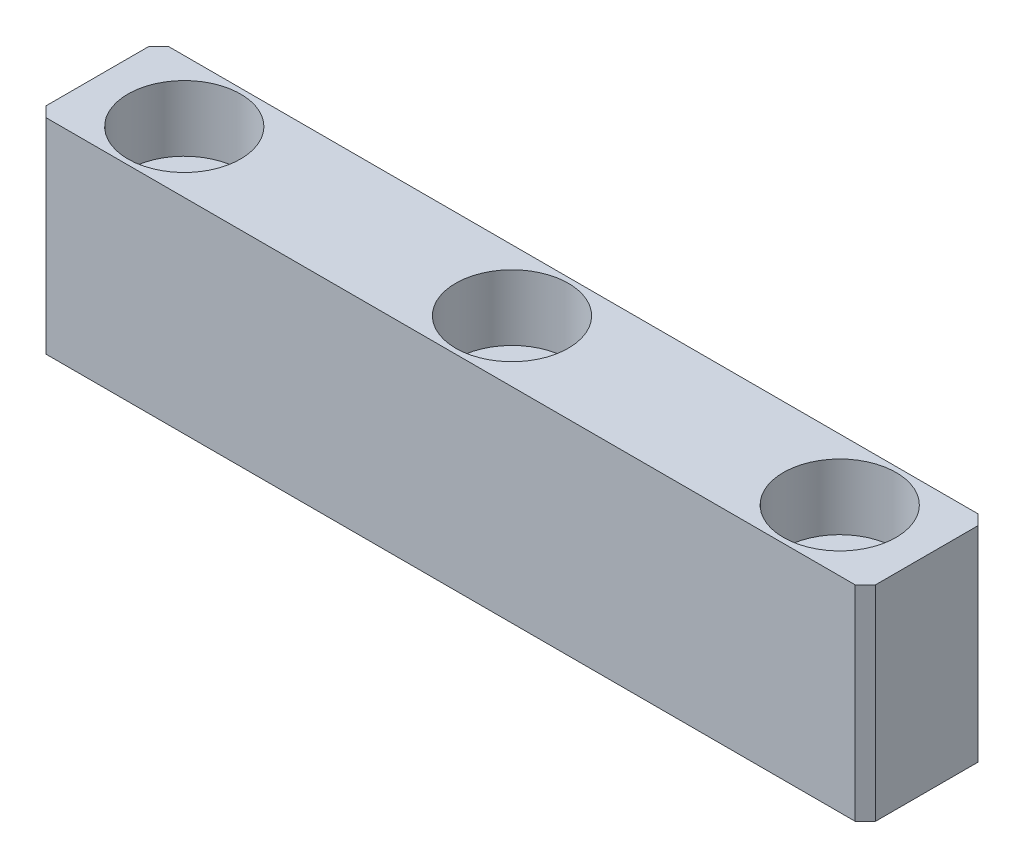
from build123d import *

# Parameters (mm, degrees)
SKETCH_1_W                   = 81
SKETCH_1_H                   = 20
EXTRUDE_1_DEPTH              = 12
HOLE_WIZARD_M6_1_D           = 6.6
HOLE_WIZARD_M6_1_CBORE_D     = 11
HOLE_WIZARD_M6_1_CBORE_DEPTH = 6.4
CHAMFER_1_SIZE               = 1


with BuildPart() as part:
    # 草图1 → 凸台-拉伸1 (new body)
    with BuildSketch(Plane.XY):
        Rectangle(SKETCH_1_W, SKETCH_1_H)
    extrude(amount=EXTRUDE_1_DEPTH)

    # M6 六角凹头螺钉的柱形沉头孔1 (through all)
    with Locations(Plane(origin=(0, 10, 0), x_dir=(1, 0, 0), z_dir=(0, 1, 0))):
        with Locations((-32, -6), (0, -6), (32, -6)):
            CounterBoreHole(HOLE_WIZARD_M6_1_D / 2, HOLE_WIZARD_M6_1_CBORE_D / 2, HOLE_WIZARD_M6_1_CBORE_DEPTH)

    # 倒角1
    chamfer_1_edges = [part.edges().sort_by_distance(p)[0] for p in [
        (-40.5, 0, 12),
        (40.5, 0, 12),
        (-40.5, 0, 0),
        (40.5, 0, 0),
    ]]
    chamfer(chamfer_1_edges, length=CHAMFER_1_SIZE)


solid = part.part
